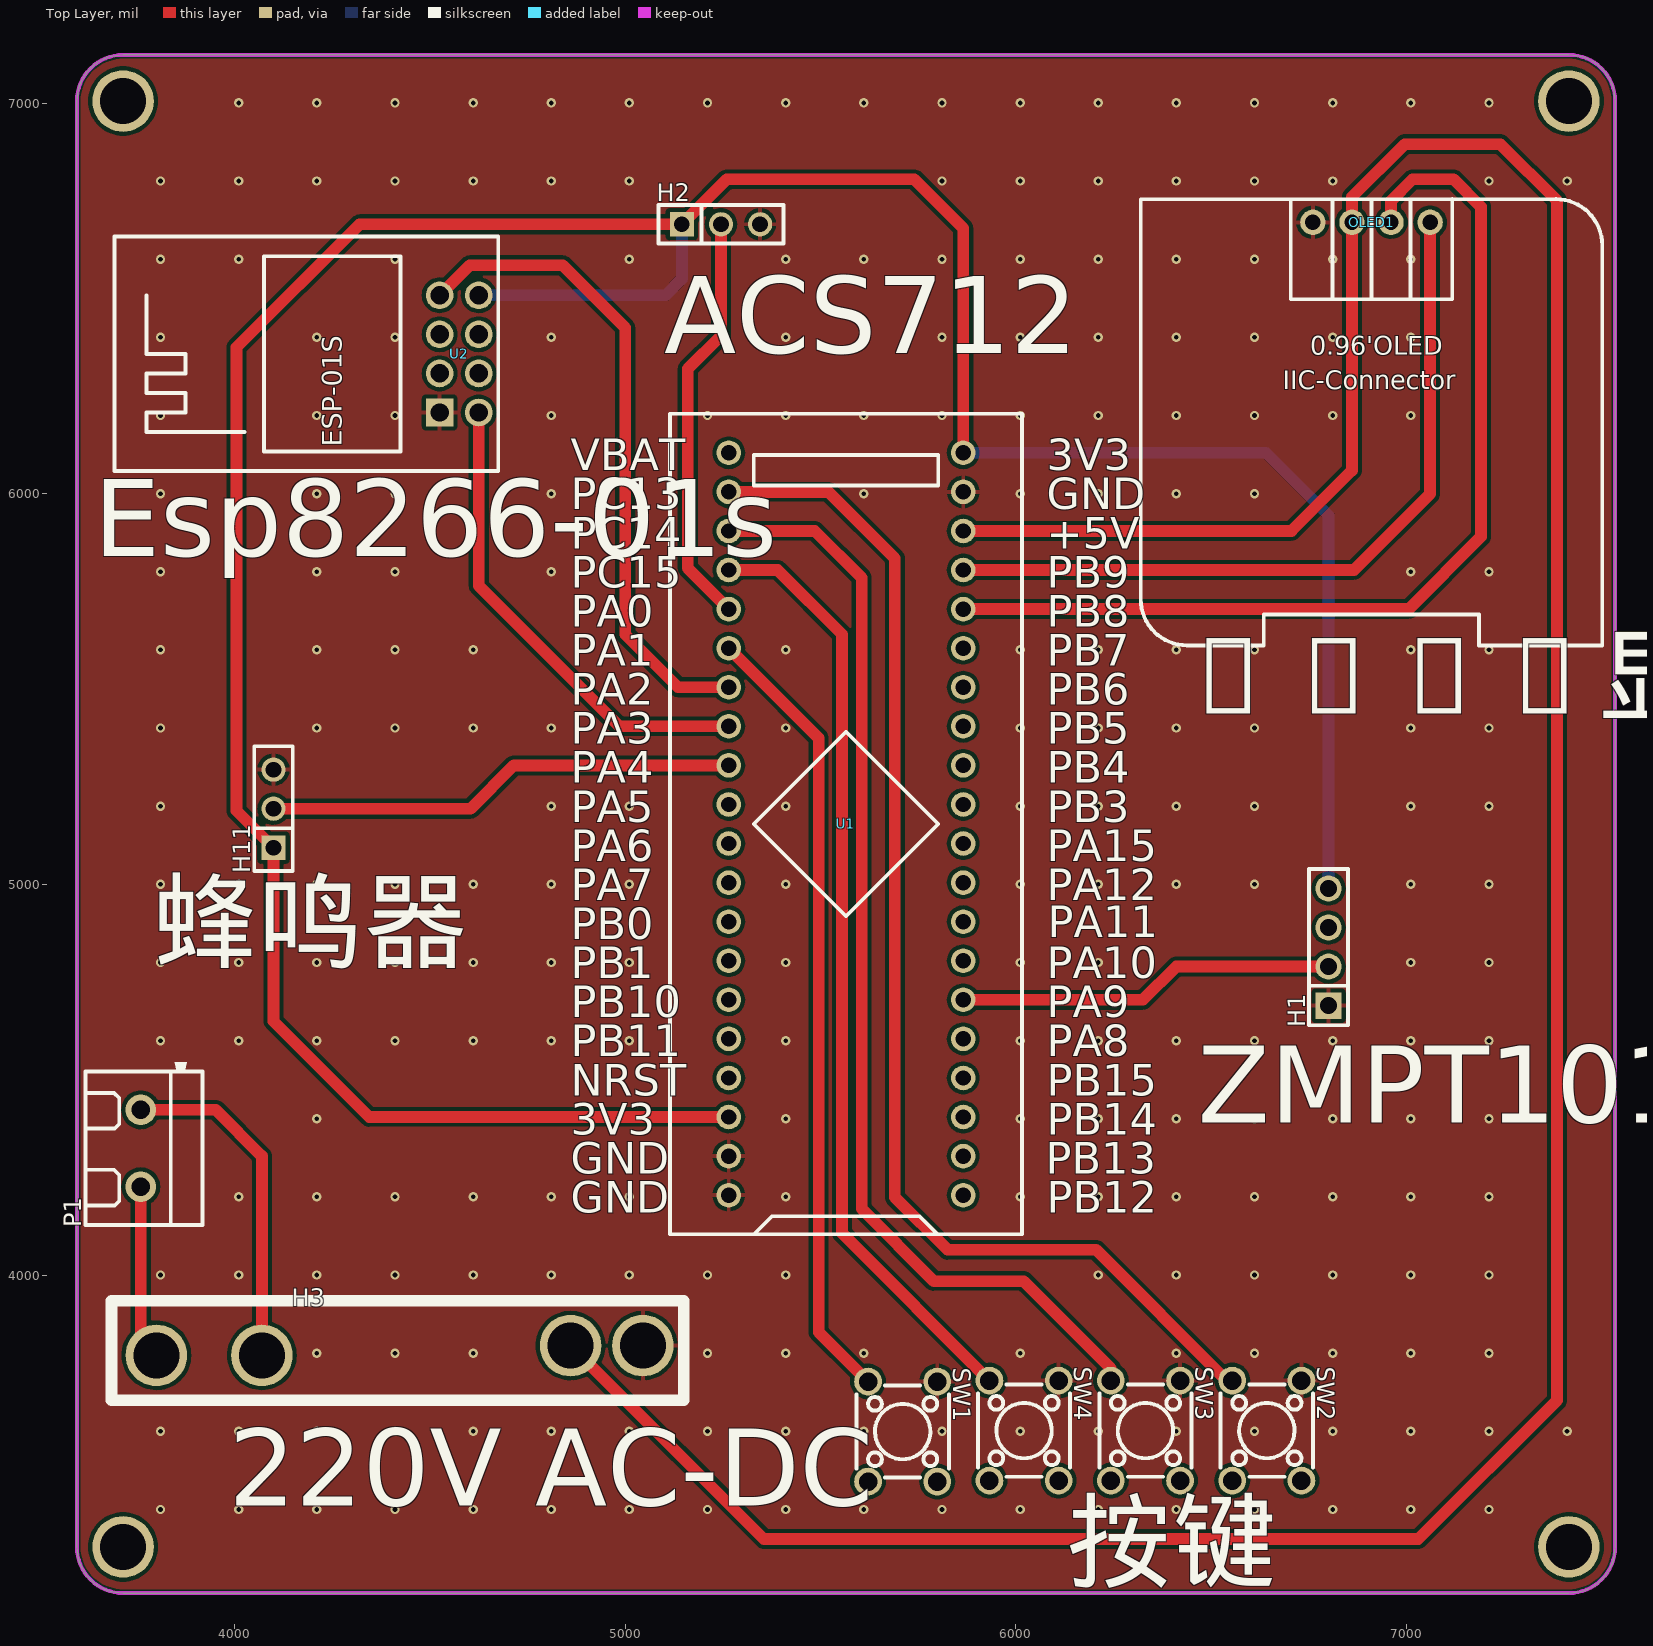
[diagram p0: Top Layer view]
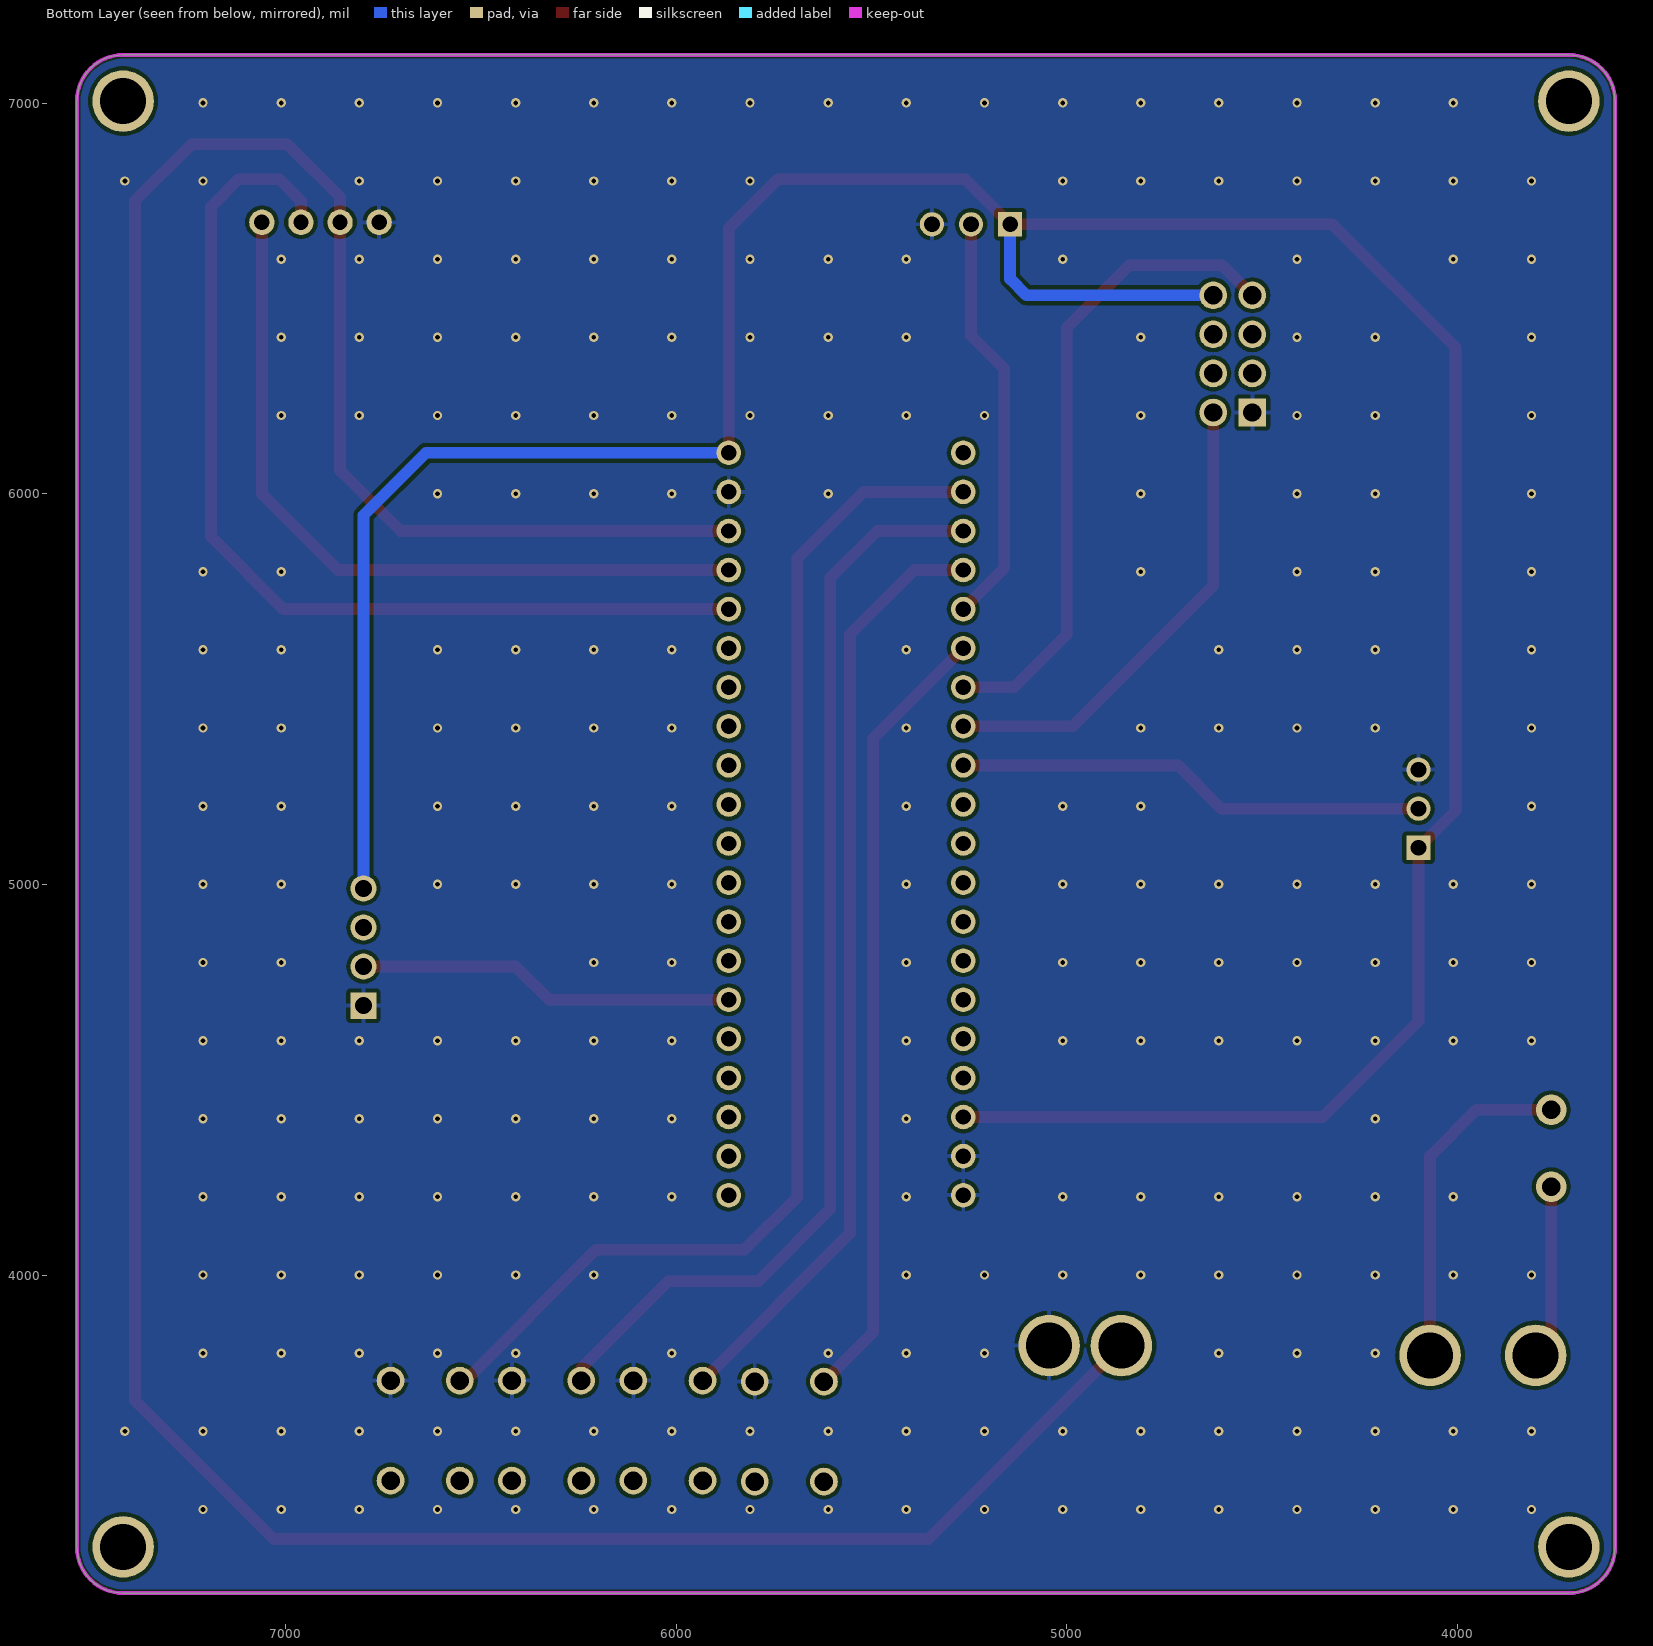
[diagram p1: Bottom Layer view, seen from below]
# Altium PCB MISC51329.pcbdoc
Units mil, origin at the board's own origin, x right, y up, seen from the top; angles counter-clockwise.
Board outline 3937.01 x 3937.01 mil, 2 copper layers (Top Layer, Bottom Layer), stack 62.206 mil thick; 12 components, 40 nets, 88 pads, 248 vias.

## Layer stack, top to bottom
Top Solder Mask Layer: solder mask 0.394, Dk 3.3
Top Layer: signal copper 1.379
Dielectric1: surface 59.449, FR4, Dk 4.5
Bottom Layer: signal copper 1.378
Bottom Solder Mask Layer: solder mask 0.394, Dk 3.3

## Board outline
3714.61,7123.5 ccw(c3714.61,7005.39) 3596.5,7005.39 3596.5,3304.61 ccw(c3714.61,3304.61) 3714.61,3186.5 7415.39,3186.5 ccw(c7415.39,3304.61) 7533.5,3304.61 7533.5,7005.39 ccw(c7415.39,7005.39) 7415.39,7123.5 3714.61,7123.5

## Design rules (kind name [scope] priority, off if disabled: settings)
BoardOutlineClearance copperThickness2oz_1 [All] p2 off: genericclearance=7.99 ignorepadtopadclearanceinfootprint=FALSE except(0: Arc-SplitContinuation Track-SplitContinuation SMDPad-SplitContinuation THPad-SplitContinuation Via-SplitContinuation Fill-SplitContinuation Region-SplitContinuation Poly-SplitContinuation Text-SplitContinuation Hole-SplitContinuation; 5.98: Arc-CutoutEdge Track-CutoutEdge SMDPad-CutoutEdge THPad-CutoutEdge Via-CutoutEdge Text-CutoutEdge; 6.9: Hole-OutlineEdge Hole-CutoutEdge; 10: Poly-OutlineEdge Poly-CutoutEdge; 11.81: Arc-OutlineEdge Track-OutlineEdge SMDPad-OutlineEdge THPad-OutlineEdge Via-OutlineEdge Fill-OutlineEdge Region-OutlineEdge Text-OutlineEdge Fill-CutoutEdge Region-CutoutEdge)
BoardOutlineClearance Plane_innerPlane_1 [All] p4 off: genericclearance=4.02 ignorepadtopadclearanceinfootprint=FALSE except(0: Arc-SplitContinuation Track-SplitContinuation SMDPad-SplitContinuation THPad-SplitContinuation Via-SplitContinuation Fill-SplitContinuation Region-SplitContinuation Poly-SplitContinuation Text-SplitContinuation Hole-SplitContinuation; 5.98: Arc-CutoutEdge Track-CutoutEdge SMDPad-CutoutEdge THPad-CutoutEdge Via-CutoutEdge Text-CutoutEdge; 6.9: Hole-OutlineEdge Hole-CutoutEdge; 10: Poly-OutlineEdge Poly-CutoutEdge; 11.81: Arc-OutlineEdge Track-OutlineEdge SMDPad-OutlineEdge THPad-OutlineEdge Via-OutlineEdge Fill-OutlineEdge Region-OutlineEdge Text-OutlineEdge Fill-CutoutEdge Region-CutoutEdge)
BoardOutlineClearance Copper_copperRegion_1 [All] p6 off: genericclearance=4.02 ignorepadtopadclearanceinfootprint=FALSE except(0: Arc-SplitContinuation Track-SplitContinuation SMDPad-SplitContinuation THPad-SplitContinuation Via-SplitContinuation Fill-SplitContinuation Region-SplitContinuation Poly-SplitContinuation Text-SplitContinuation Hole-SplitContinuation; 5.98: Arc-CutoutEdge Track-CutoutEdge SMDPad-CutoutEdge THPad-CutoutEdge Via-CutoutEdge Text-CutoutEdge; 6.9: Hole-OutlineEdge Hole-CutoutEdge; 10: Poly-OutlineEdge Poly-CutoutEdge; 11.81: Arc-OutlineEdge Track-OutlineEdge SMDPad-OutlineEdge THPad-OutlineEdge Via-OutlineEdge Fill-OutlineEdge Region-OutlineEdge Text-OutlineEdge Fill-CutoutEdge Region-CutoutEdge)
BoardOutlineClearance copperThickness1oz_1 [All] p8: genericclearance=4.02 ignorepadtopadclearanceinfootprint=FALSE except(0: Arc-SplitContinuation Track-SplitContinuation SMDPad-SplitContinuation THPad-SplitContinuation Via-SplitContinuation Fill-SplitContinuation Region-SplitContinuation Poly-SplitContinuation Text-SplitContinuation Hole-SplitContinuation; 5.98: Arc-CutoutEdge Track-CutoutEdge SMDPad-CutoutEdge THPad-CutoutEdge Via-CutoutEdge Text-CutoutEdge; 6.9: Hole-OutlineEdge Hole-CutoutEdge; 10: Poly-OutlineEdge Poly-CutoutEdge; 11.81: Arc-OutlineEdge Track-OutlineEdge SMDPad-OutlineEdge THPad-OutlineEdge Via-OutlineEdge Fill-OutlineEdge Region-OutlineEdge Text-OutlineEdge Fill-CutoutEdge Region-CutoutEdge)
Clearance copperThickness2oz [All] p1 off: gap=7.99 ignorepadtopadclearanceinfootprint=FALSE except(5.98: SMDPad-Track SMDPad-SMDPad THPad-Track SMDPad-THPad THPad-THPad Track-Via SMDPad-Via THPad-Via Via-Via Fill-SMDPad Region-SMDPad Fill-THPad Region-THPad Fill-Via Region-Via Fill-Fill Fill-Region Region-Region Arc-Track Arc-SMDPad Arc-THPad Arc-Via Fill-Arc Region-Arc Arc-Arc Text-Track SMDPad-Text Text-THPad Text-Via Fill-Text Region-Text Arc-Text Text-Text; 6.9: Hole-Track Hole-SMDPad Hole-THPad Hole-Via Fill-Hole Region-Hole Hole-Arc Hole-Text; 10: Poly-Track Poly-SMDPad Poly-THPad Poly-Via Poly-Fill Poly-Region Poly-Poly Poly-Arc Poly-Text Poly-Hole; 11.81: Fill-Track Region-Track)
Clearance Plane_innerPlane [All] p3 off: gap=4.02 ignorepadtopadclearanceinfootprint=FALSE except(5.98: SMDPad-Track SMDPad-SMDPad THPad-Track SMDPad-THPad THPad-THPad Track-Via SMDPad-Via THPad-Via Via-Via Fill-SMDPad Region-SMDPad Fill-THPad Region-THPad Fill-Via Region-Via Fill-Fill Fill-Region Region-Region Arc-Track Arc-SMDPad Arc-THPad Arc-Via Fill-Arc Region-Arc Arc-Arc Text-Track SMDPad-Text Text-THPad Text-Via Fill-Text Region-Text Arc-Text Text-Text; 6.9: Hole-Track Hole-SMDPad Hole-THPad Hole-Via Fill-Hole Region-Hole Hole-Arc Hole-Text; 10: Poly-Track Poly-SMDPad Poly-THPad Poly-Via Poly-Fill Poly-Region Poly-Poly Poly-Arc Poly-Text Poly-Hole; 11.81: Fill-Track Region-Track)
Clearance Copper_copperRegion [All] p5 off: gap=4.02 ignorepadtopadclearanceinfootprint=FALSE except(5.98: SMDPad-Track SMDPad-SMDPad THPad-Track SMDPad-THPad THPad-THPad Track-Via SMDPad-Via THPad-Via Via-Via Fill-SMDPad Region-SMDPad Fill-THPad Region-THPad Fill-Via Region-Via Fill-Fill Fill-Region Region-Region Arc-Track Arc-SMDPad Arc-THPad Arc-Via Fill-Arc Region-Arc Arc-Arc Text-Track SMDPad-Text Text-THPad Text-Via Fill-Text Region-Text Arc-Text Text-Text; 6.9: Hole-Track Hole-SMDPad Hole-THPad Hole-Via Fill-Hole Region-Hole Hole-Arc Hole-Text; 10: Poly-Track Poly-SMDPad Poly-THPad Poly-Via Poly-Fill Poly-Region Poly-Poly Poly-Arc Poly-Text Poly-Hole; 11.81: Fill-Track Region-Track)
Clearance copperThickness1oz [All] p7: gap=4.02 ignorepadtopadclearanceinfootprint=FALSE except(5.98: SMDPad-Track SMDPad-SMDPad THPad-Track SMDPad-THPad THPad-THPad Track-Via SMDPad-Via THPad-Via Via-Via Fill-SMDPad Region-SMDPad Fill-THPad Region-THPad Fill-Via Region-Via Fill-Fill Fill-Region Region-Region Arc-Track Arc-SMDPad Arc-THPad Arc-Via Fill-Arc Region-Arc Arc-Arc Text-Track SMDPad-Text Text-THPad Text-Via Fill-Text Region-Text Arc-Text Text-Text; 6.9: Hole-Track Hole-SMDPad Hole-THPad Hole-Via Fill-Hole Region-Hole Hole-Arc Hole-Text; 10: Poly-Track Poly-SMDPad Poly-THPad Poly-Via Poly-Fill Poly-Region Poly-Poly Poly-Arc Poly-Text Poly-Hole; 11.81: Fill-Track Region-Track)
DiffPairsRouting differentialPair [All] p1: maxlimit=6 minlimit=6 mostfreqgap=6 toplayer_minwidth=5 toplayer_prefwidth=10 toplayer_maxwidth=100 toplayer_mingap=6 toplayer_prefgap=6 toplayer_maxgap=6 bottomlayer_minwidth=5 bottomlayer_prefwidth=10 bottomlayer_maxwidth=100 bottomlayer_mingap=6 bottomlayer_prefgap=6 bottomlayer_maxgap=6 maxuncoupledlength=10
HoleToHoleClearance otherClearance [All] p1: gap=11.81 allowstackedmicrovias=TRUE
Length netLength [All] p1: minlimit=0 maxlimit=0
PasteMaskExpansion pasteMaskExpansion [All] p1: expansion=0
PlaneConnect innerPlane [All] p1: planeconnectstyle=Relief reliefexpansion=20 reliefentries=4 reliefconductorwidth=10 reliefairgap=10
PolygonConnect copperRegion [All] p1: connectstyle=Relief reliefconductorwidth=10 reliefentries=4 polygonreliefangle="90 Angle" airgapwidth=10 via.connectstyle=Relief via.reliefconductorwidth=10 via.reliefentries=4 via.polygonreliefangle="90 Angle" via.airgapwidth=10
RoutingVias viaSize [All] p1: holewidth=12.01 width=24.02 viastyle="Through Hole" minholewidth=11.81 minwidth=19.68 maxholewidth=248.03 maxwidth=393.7
SolderMaskExpansion solderMaskExpansion [IsVia] p1: expansion=-1000 istentingtop=TRUE
SolderMaskExpansion solderMaskExpansion [All] p2: expansion=2 istentingtop=FALSE
Width copperThickness2oz_2 [All] p1 off: maxlimit=100 minlimit=8 preferedwidth=10
Width copperThickness1oz_2 [All] p2: maxlimit=100 minlimit=5 preferedwidth=10

## Components (designator, comment, footprint, x,y, rotation, side; value= is the part's Value field where it differs from the comment)
H1 "" HDR-TH_4P-P2.54-V-M 6800,4840 r90 top
H2 "" HDR-TH_3P-P2.54-V-F 5245,6690 r0 top
H3 "" HDR-TH_4P-P2.54-V-F 4345,3820 r0 top
H11 "" HDR-TH_3P-P2.54-V-F 4099.74,5194.14 r90 top
OLED1 "" 0.96OLED_4P 6910,6695 r0 top
P1 "KF301-2P接线端子" CONN-TH_XY301V-A-5.0-2P 3760,4325 r90 top
SW1 "" SW-TH_4P-L6.0-W6.0-P4.50-LS6.5 5710,3600 r270 top
SW2 "" SW-TH_4P-L6.0-W6.0-P4.50-LS6.5 6642.14,3602.47 r270 top
SW3 "" SW-TH_4P-L6.0-W6.0-P4.50-LS6.5 6331.43,3602.47 r270 top
SW4 "" SW-TH_4P-L6.0-W6.0-P4.50-LS6.5 6020.71,3602.47 r270 top
U1 "STM32F103C8T6-Card" CONN-TH_L53.3-W22.9_STM32F103C8T6-CARD 5565,5155 r90 top
U2 "ESP-01S" WIFIM-TH_ESP-01S 4575,6358.21 r90 top

## Footprints (in the part's own frame and the unit in brackets; to place one, negate y for a bottom-side part, rotate by r counter-clockwise, add the part's x,y. Pads: shape width x height; smd on the part's side, far side on the other; paste and mask are expansions set on the pad)
0.96OLED_4P [mm]
  round 1.65 hole 1 copper offset 0,0: 1(-3.81,-0.001) 2(-1.27,0.002) 3(1.27,0.002) 4(3.81,0.002)
  silkscreen extent -15,-27.5 15,1.5
CONN-TH_L53.3-W22.9_STM32F103C8T6-CARD [mm]
  round 1.6 hole 1: 1(-24.13,-7.62) 2(-21.59,-7.62) 3(-19.05,-7.62) 4(-16.51,-7.62) 5(-13.97,-7.62) 6(-11.43,-7.62) 7(-8.89,-7.62) 8(-6.35,-7.62) 9(-3.81,-7.62) 10(-1.27,-7.62) 11(1.27,-7.62) 12(3.81,-7.62) 13(6.35,-7.62) 14(8.89,-7.62) 15(11.43,-7.62) 16(13.97,-7.62) 17(16.51,-7.62) 18(19.05,-7.62) 19(21.59,-7.62) 20(24.13,-7.62) 21(24.13,7.62) 22(21.59,7.62) 23(19.05,7.62) 24(16.51,7.62) 25(13.97,7.62) 26(11.43,7.62) 27(8.89,7.62) 28(6.35,7.62) 29(3.81,7.62) 30(1.27,7.62) 31(-1.27,7.62) 32(-3.81,7.62) 33(-6.35,7.62) 34(-8.89,7.62) 35(-11.43,7.62) 36(-13.97,7.62) 37(-16.51,7.62) 38(-19.05,7.62) 39(-21.59,7.62) 40(-24.13,7.62)
  silkscreen extent -26.67,-11.43 26.67,11.43
CONN-TH_XY301V-A-5.0-2P [mm]
  round 2 hole 1.2: 1(-2.5,0) 2(2.5,0)
  silkscreen extent -5,-4 5.6,3.6
HDR-TH_3P-P2.54-V-F [mil]
  rect 62x62 hole 40.16: 1(-100,0)
  round 62 hole 40.16: 2(0,0) 3(100,0)
  silkscreen extent -160,-49 160,49
HDR-TH_4P-P2.54-V-F [mm]
  round 4 hole 3: 1(-13.843,-0.635) 2(-6.985,-0.635) 3(13.081,0) 4(17.78,0)
HDR-TH_4P-P2.54-V-M [mm]
  rect 1.7x1.7 hole 1.1: 1(-3.81,0)
  round 1.7 hole 1.1: 2(-1.27,0) 3(1.27,0) 4(3.81,0)
  silkscreen extent -5.08,-1.27 5.08,1.27
SW-TH_4P-L6.0-W6.0-P4.50-LS6.5 [mm]
  round 1.8 hole 1.2: 1(-3.25,2.25) 2(3.25,2.25) 3(-3.25,-2.25) 4(3.25,-2.25)
  silkscreen extent -3,-3 3,3
WIFIM-TH_ESP-01S [mm]
  rect 1.8x1.8 hole 1.2: 1(-3.81,1.27)
  round 1.8 hole 1.2: 2(-1.27,1.27) 3(1.27,1.27) 4(3.81,1.27) 5(3.81,-1.27) 6(1.27,-1.27) 7(-1.27,-1.27) 8(-3.81,-1.27)
  silkscreen extent -7.62,-2.54 7.62,22.4

## Free pads (board coordinates)
  round 157.48 hole 118.11: 1(3714.61,7005.39) 1(3714.61,3304.61) 1(7415.39,7005.39) 1(7415.39,3304.61)

## Via types
v1: diameter 24.02, hole 12, Top Layer to Bottom Layer, 248 vias

## Nets (pads, with @x,y where several pads share a name; then routed paths per layer and width w, separated by ;. In a path a pad name is that pad's centre, name@x,y a point inside that pad or via, vN(x,y) a via of type N, cw(c..) or ccw(c..) an arc to the next point about the centre after c; other vN are vias at no path point)
10: H1.3
$1N17128: H3.1 P1.1 | length 448.1
  Top Layer w30: P1.1 3760,3835 H3.1
$1N17129: H3.2 P1.2 | length 869.1
  Top Layer w30: P1.2 3951.57,4423.43 4070,4305 H3.2
+5V: H3.3 OLED1.2 U1.18 | length 8347.3
  Top Layer w30: H3.3 5355,3325 7030,3325 7385,3680 7385,6750 7240,6895 6995,6895 6860,6760 6860,6695.05 6860,6060 6705,5905 U1.18
GND: H1.1 H2.3 H3.4 H11.3 OLED1.1 SW1.1 SW2.1 SW3.1 SW4.1 U1.19 U1.39 U1.40 U2.1
  other v1: 3810.6,3400.6 4010.6,3400.6 4210.6,3400.6 4410.6,3400.6 4610.6,3400.6 4810.6,3400.6 5010.6,3400.6 5210.6,3400.6 5410.6,3400.6 5610.6,3400.6 5810.6,3400.6 6010.6,3400.6 6210.6,3400.6 6410.6,3400.6 6610.6,3400.6 6810.6,3400.6 7010.6,3400.6 7210.6,3400.6 3810.6,3600.6 4010.6,3600.6 4210.6,3600.6 4410.6,3600.6 4610.6,3600.6 4810.6,3600.6 5010.6,3600.6 5210.6,3600.6 5410.6,3600.6 5610.6,3600.6 5810.6,3600.6 6010.6,3600.6 6210.6,3600.6 6410.6,3600.6 6610.6,3600.6 6810.6,3600.6 7010.6,3600.6 7210.6,3600.6 7410.6,3600.6 4210.6,3800.6 4410.6,3800.6 4610.6,3800.6 5210.6,3800.6 5410.6,3800.6 5610.6,3800.6 6010.6,3800.6 6410.6,3800.6 6610.6,3800.6 6810.6,3800.6 7010.6,3800.6 7210.6,3800.6 3810.6,4000.6 4010.6,4000.6 4210.6,4000.6 4410.6,4000.6 4610.6,4000.6 4810.6,4000.6 5010.6,4000.6 5210.6,4000.6 5410.6,4000.6 6210.6,4000.6 6410.6,4000.6 6610.6,4000.6 6810.6,4000.6 7010.6,4000.6 7210.6,4000.6 4010.6,4200.6 4210.6,4200.6 4410.6,4200.6 4610.6,4200.6 4810.6,4200.6 5010.6,4200.6 5410.6,4200.6 6010.6,4200.6 6210.6,4200.6 6410.6,4200.6 6610.6,4200.6 6810.6,4200.6 7010.6,4200.6 7210.6,4200.6 4210.6,4400.6 5410.6,4400.6 6010.6,4400.6 6210.6,4400.6 6410.6,4400.6 6610.6,4400.6 6810.6,4400.6 7010.6,4400.6 7210.6,4400.6 3810.6,4600.6 4010.6,4600.6 4210.6,4600.6 4410.6,4600.6 4610.6,4600.6 4810.6,4600.6 5010.6,4600.6 5410.6,4600.6 6010.6,4600.6 6210.6,4600.6 6410.6,4600.6 6610.6,4600.6 6810.6,4600.6 7010.6,4600.6 7210.6,4600.6 3810.6,4800.6 4010.6,4800.6 4210.6,4800.6 4410.6,4800.6 4610.6,4800.6 4810.6,4800.6 5010.6,4800.6 5410.6,4800.6 6010.6,4800.6 6210.6,4800.6 7010.6,4800.6 7210.6,4800.6 3810.6,5000.6 4010.6,5000.6 4210.6,5000.6 4410.6,5000.6 4610.6,5000.6 4810.6,5000.6 5010.6,5000.6 5410.6,5000.6 6010.6,5000.6 6210.6,5000.6 6410.6,5000.6 6610.6,5000.6 7010.6,5000.6 7210.6,5000.6 3810.6,5200.6 4810.6,5200.6 5010.6,5200.6 5410.6,5200.6 6010.6,5200.6 6210.6,5200.6 6410.6,5200.6 6610.6,5200.6 7010.6,5200.6 7210.6,5200.6 3810.6,5400.6 4210.6,5400.6 4410.6,5400.6 4610.6,5400.6 4810.6,5400.6 5410.6,5400.6 6010.6,5400.6 6210.6,5400.6 6410.6,5400.6 6610.6,5400.6 7010.6,5400.6 7210.6,5400.6 3810.6,5600.6 4210.6,5600.6 4410.6,5600.6 4610.6,5600.6 5410.6,5600.6 6010.6,5600.6 6210.6,5600.6 6410.6,5600.6 6610.6,5600.6 7010.6,5600.6 7210.6,5600.6 3810.6,5800.6 4210.6,5800.6 4410.6,5800.6 4810.6,5800.6 7010.6,5800.6 7210.6,5800.6 3810.6,6000.6 4210.6,6000.6 4410.6,6000.6 4810.6,6000.6 5610.6,6000.6 6010.6,6000.6 6210.6,6000.6 6410.6,6000.6 6610.6,6000.6 3810.6,6200.6 4210.6,6200.6 4410.6,6200.6 4810.6,6200.6 5210.6,6200.6 5410.6,6200.6 5610.6,6200.6 5810.6,6200.6 6010.6,6200.6 6210.6,6200.6 6410.6,6200.6 6610.6,6200.6 6810.6,6200.6 7010.6,6200.6 3810.6,6400.6 4210.6,6400.6 4410.6,6400.6 4810.6,6400.6 5410.6,6400.6 5610.6,6400.6 5810.6,6400.6 6010.6,6400.6 6210.6,6400.6 6410.6,6400.6 6610.6,6400.6 6810.6,6400.6 7010.6,6400.6 3810.6,6600.6 4010.6,6600.6 4410.6,6600.6 5010.6,6600.6 5410.6,6600.6 5610.6,6600.6 5810.6,6600.6 6010.6,6600.6 6210.6,6600.6 6410.6,6600.6 6610.6,6600.6 6810.6,6600.6 7010.6,6600.6 3810.6,6800.6 4010.6,6800.6 4210.6,6800.6 4410.6,6800.6 4610.6,6800.6 4810.6,6800.6 5010.6,6800.6 5810.6,6800.6 6010.6,6800.6 6210.6,6800.6 6410.6,6800.6 6610.6,6800.6 6810.6,6800.6 7210.6,6800.6 7410.6,6800.6 4010.6,7000.6 4210.6,7000.6 4410.6,7000.6 4610.6,7000.6 4810.6,7000.6 5010.6,7000.6 5210.6,7000.6 5410.6,7000.6 5610.6,7000.6 5810.6,7000.6 6010.6,7000.6 6210.6,7000.6 6410.6,7000.6 6610.6,7000.6 6810.6,7000.6 7010.6,7000.6 7210.6,7000.6
NRST: U1.37
PA0: H2.2 U1.25 | length 1063.7
  Top Layer w30: H2.2 5245,6405 5160,6320 5160,5810 U1.25
PA1: SW1.3 U1.26 | length 2024.7
  Top Layer w30: U1.26 5495,5375 5495,3854.37 SW1.3
PA2: U1.27 U2.4 | length 1679
  Top Layer w30: U2.4 4601.79,6585 4840,6585 5000,6425 5000,5640 5135,5505 U1.27
PA3: U1.28 U2.8 | length 1232.3
  Top Layer w30: U2.8 4625,5765 4985,5405 U1.28
PA4: H11.2 U1.29 | length 1211.2
  Top Layer w30: H11.2 4604.14,5194.14 4715,5305 U1.29
PA5: U1.30
PA6: U1.31
PA7: U1.32
PA8: U1.5
PA9: H1.2 U1.6 | length 970.2
  Top Layer w30: U1.6 6325,4705 6410,4790 H1.2
PA10: U1.7
PA11: U1.8
PA12: U1.9
PA15: U1.10
PB0: U1.33
PB1: U1.34
PB3: U1.11
PB4: U1.12
PB5: U1.13
PB6: U1.14
PB7: U1.15
PB8: OLED1.3 U1.16 | length 2583.4
  Top Layer w30: U1.16 7005,5705 7190,5890 7190,6735 7120,6805 7015,6805 6960,6750 OLED1.3@6960,6695.05
PB9: OLED1.4 U1.17 | length 1970.8
  Top Layer w30: U1.17 6865,5805 7060,6000 OLED1.4@7060,6695.05
PB10: U1.35
PB11: U1.36
PB12: U1.1
PB13: U1.2
PB14: U1.3
PB15: U1.4
PC13: SW2.3 U1.22 | length 3188.5
  Top Layer w30: U1.22 5520,6005 5690,5835 5690,4200 5825,4065 6205,4065 6539.58,3730.42 SW2.3
PC14: SW3.3 U1.23 | length 2843.2
  Top Layer w30: U1.23 5485,5905 5605,5785 5605,4170 5790,3985 6020,3985 6242.85,3762.15 SW3.3
PC15: SW4.3 U1.24 | length 2424.1
  Top Layer w30: U1.24 5390,5805 5555,5640 5555,4107.55 SW4.3
VBAT: U1.21
VCC: H1.4 H2.1 H11.1 U1.20 U1.38 U2.5 | length 8329.3
  Top Layer w30: U1.38 4345,4405 4099.74,4650.26 H11.1 4005,5188.88 4005,6375 4320,6690 H2.1 5260,6805 5740,6805 5865,6680 U1.20
  Bottom Layer w30: U2.5 5103.21,6508.21 5145,6550 H2.1 ; U1.20 6640,6105 6800,5945 H1.4
pads on no net: SW1.2 SW1.4 SW2.2 SW2.4 SW3.2 SW3.4 SW4.2 SW4.4 U2.2 U2.3 U2.6 U2.7

## Polygon pours and split planes (outlines as drawn)
GND on Bottom Layer (solid, remove dead copper, pour order 2): 3525,7245 3525,3080 7700,3080 7700,7245
GND on Top Layer (solid, remove dead copper, pour order 2): 3000,7415 3000,3000 7930,3000 7930,7415

## Keep-outs
Board Outline Layer:
  the board outline again, w10

## Silkscreen, mask and mechanical layers (free items; w line width, h text height)
Top Silkscreen Layer:
  lines w30: 3685,3680 3685,3935 5150,3935 5150,3680 3685,3680
  text "ACS712" at 5100,6360 h196.85
  text "VBAT" at 4860.95,6060 h80
  text "3V3" at 6079.16,6060 h80
  text "PC13" at 4860.95,5960 h80
  text "GND" at 6079.16,5960 h80
  text "PC14" at 4860.95,5860 h80
  text "+5V" at 6079.16,5860 h80
  text "Esp8266-01s" at 3640,5840 h196.85
  text "PC15" at 4860.95,5760 h80
  text "PB9" at 6079.16,5760 h80
  text "PA0" at 4860.95,5660 h80
  text "PB8" at 6079.16,5660 h80
  text "PA1" at 4860.95,5560 h80
  text "PB7" at 6079.16,5560 h80
  text "PA2" at 4860.95,5460 h80
  text "PB6" at 6079.16,5460 h80
  text "Oled显示器" at 6408.66,5436.57 h196.85
  text "PA3" at 4860.95,5360 h80
  text "PB5" at 6079.16,5360 h80
  text "PA4" at 4860.95,5260 h80
  text "PB4" at 6079.16,5260 h80
  text "PA5" at 4860.95,5160 h80
  text "PB3" at 6079.16,5160 h80
  text "PA6" at 4860.95,5060 h80
  text "PA15" at 6079.16,5060 h80
  text "PA7" at 4860.95,4960 h80
  text "PA12" at 6079.16,4960 h80
  text "PA11" at 6080.95,4865 h80
  text "PB0" at 4860.95,4860 h80
  text "蜂鸣器" at 3790,4810 h196.85
  text "PB1" at 4860.95,4760 h80
  text "PA10" at 6079.16,4760 h80
  text "PB10" at 4860.95,4660 h80
  text "PA9" at 6079.16,4660 h80
  text "PB11" at 4860.95,4560 h80
  text "PA8" at 6079.16,4560 h80
  text "NRST" at 4860.95,4460 h80
  text "PB15" at 6079.16,4460 h80
  text "ZMPT101B" at 6465,4390 h196.85
  text "3V3" at 4860.95,4360 h80
  text "PB14" at 6079.16,4360 h80
  text "GND" at 4860.95,4260 h80
  text "PB13" at 6075.95,4260 h80
  text "GND" at 4860.95,4160 h80
  text "PB12" at 6079.16,4160 h80
  text "220V AC-DC" at 3985,3410 h196.85
  text "按键" at 6130,3225 h196.85